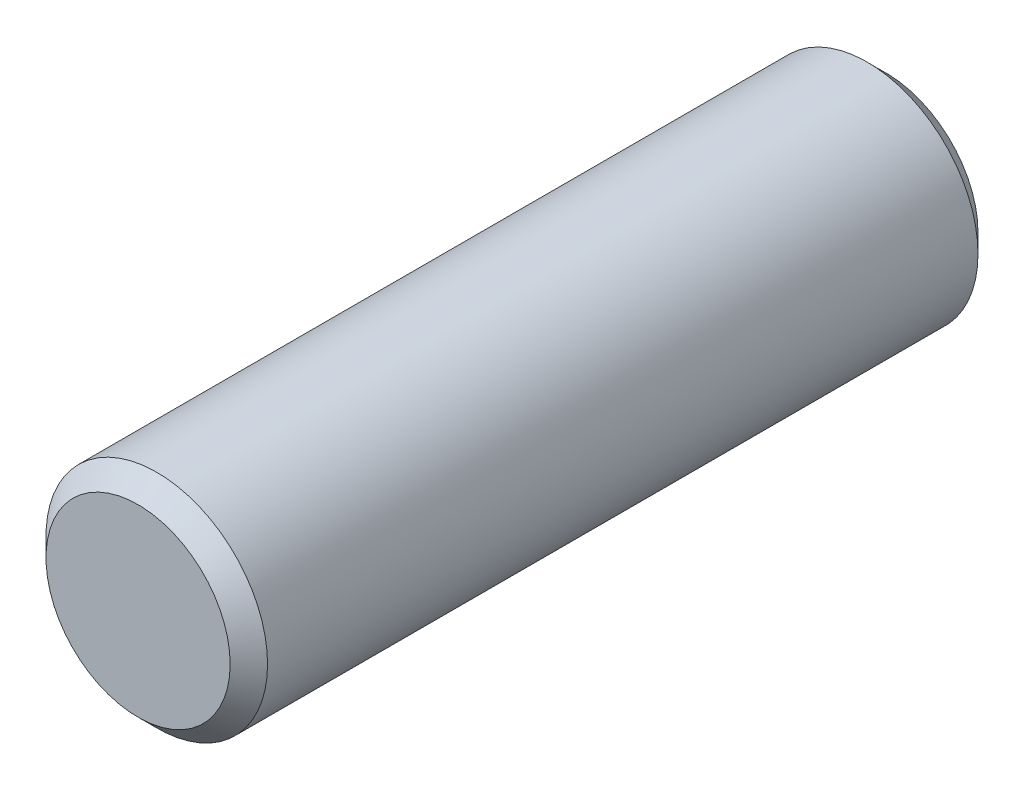
from build123d import *

# Parameters (mm, degrees)
SKETCH1_R           = 5.925
BOSS_EXTRUDE1_DEPTH = 40
CHAMFER1_SIZE       = 1


with BuildPart() as part:
    # Sketch1 → Boss-Extrude1 (new body)
    with BuildSketch(Plane.XY):
        Circle(SKETCH1_R)
    extrude(amount=BOSS_EXTRUDE1_DEPTH)

    # Chamfer1
    chamfer1_edges = [part.edges().sort_by_distance(p)[0] for p in [
        (-5.925, 0, 0),
        (-5.925, 0, 40),
    ]]
    chamfer(chamfer1_edges, length=CHAMFER1_SIZE)


solid = part.part
